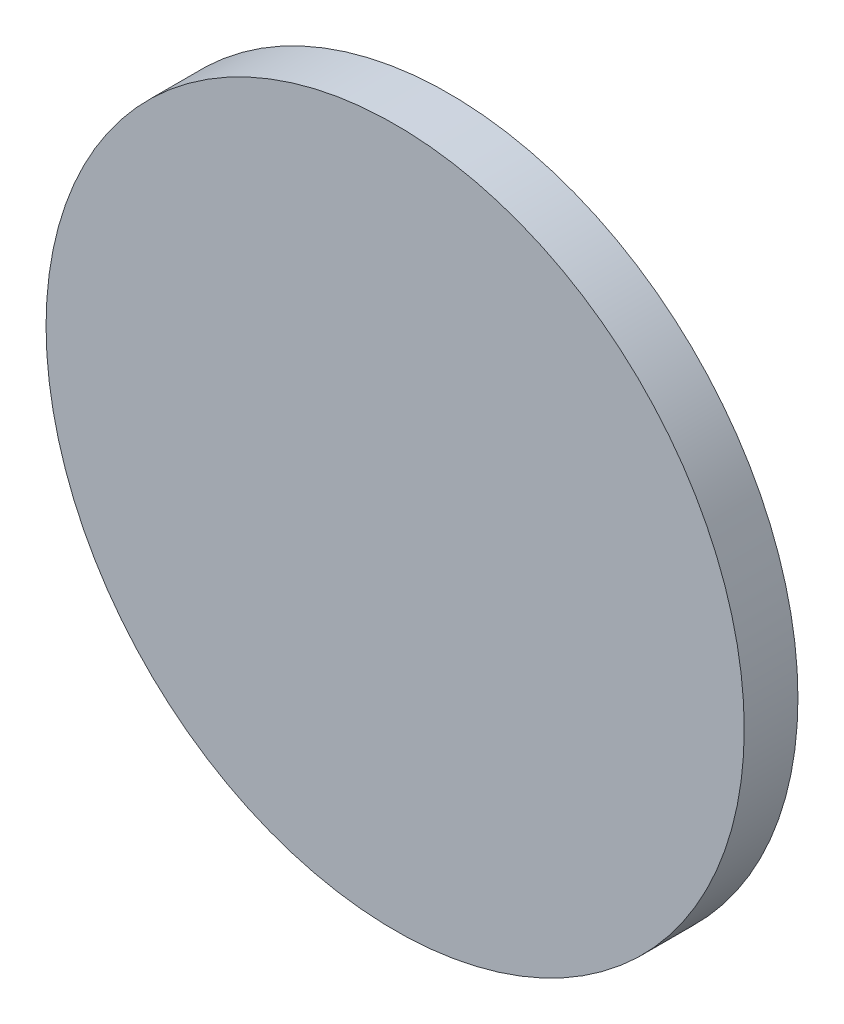
SolidWorks part; units mm, degrees
material "普通碳钢"
ref_plane "Front Plane" through (0, 0, 0) normal (0, 0, 1) x (1, 0, 0)
ref_plane "Top Plane" through (0, 0, 0) normal (0, 1, 0) x (1, 0, 0)
ref_plane "Right Plane" through (0, 0, 0) normal (1, 0, 0) x (0, 0, -1)
sketch "Sketch1" plane through (0, 0, 0) normal (0, 0, 1) x (1, 0, 0)
  circle A0 centre (0, 0) radius 65
  dimension "D1" = 130
extrude "Boss-Extrude1" add sketch "Sketch1" along normal blind 10
